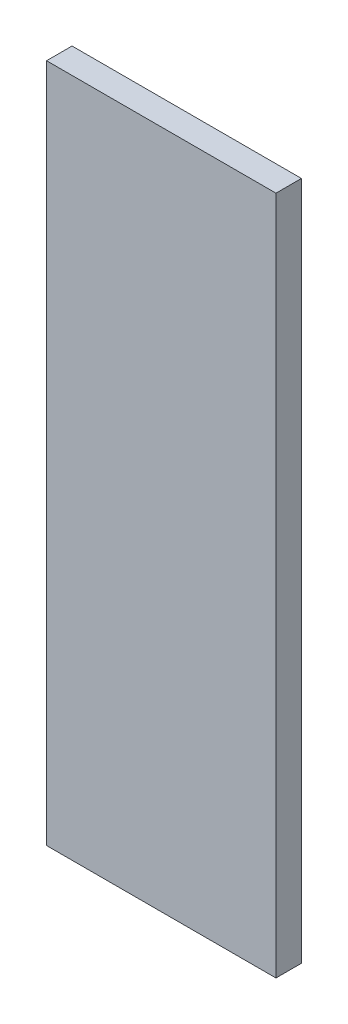
SolidWorks part; units mm, degrees
ref_plane "前视基准面" through (0, 0, 0) normal (0, 0, 1) x (1, 0, 0)
ref_plane "上视基准面" through (0, 0, 0) normal (0, 1, 0) x (1, 0, 0)
ref_plane "右视基准面" through (0, 0, 0) normal (1, 0, 0) x (0, 0, -1)
sketch "草图1" plane through (0, 0, 0) normal (0, 0, 1) x (1, 0, 0)
  line L0 (-34.9565, 21.9783) -> (-7.9565, 21.9783)
  line L5 (-34.9565, -58.0217) -> (-34.9565, 21.9783)
  line L6 (-34.9565, -58.0217) -> (-7.9565, -58.0217)
  line L7 (-7.9565, -58.0217) -> (-7.9565, 21.9783)
  dimension "D1" = 27
  dimension "D2" = 80
extrude "凸台-拉伸2" add sketch "草图1" along normal blind 3 contours L5 L0 L7 L6
extrude "切除-拉伸1" cut sketch "草图2" against normal blind 15
sketch "草图2" plane through (820.1041, -68.0217, 1111.2312) normal (0, -1, 0) x (-0.9925, 0, -0.1219)
  line L0 (957.1306, 1000.5442) -> (983.9293, 997.2537) construction
  line L3 (955.5463, 987.6411) -> (982.345, 984.3506) construction
  circle A0 centre (963.0859, 999.813) radius 1
  circle A1 centre (977.9741, 997.9849) radius 1
  circle A2 centre (961.5016, 986.9099) radius 1
  circle A3 centre (976.3898, 985.0818) radius 1
sketch "草图3" plane through (0, -58.0217, 0) normal (0, -1, 0) x (1, 0, 0)
  circle A0 centre (-28.9565, 1.5) radius 1
  circle A1 centre (-13.9565, 1.5) radius 1
